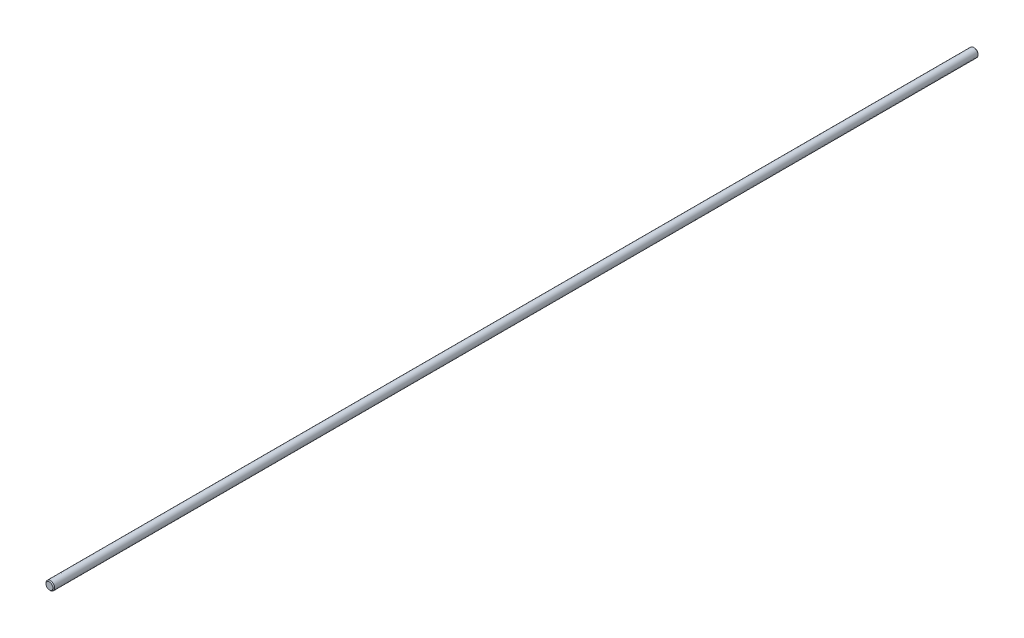
SolidWorks part; units mm, degrees
material "45#"
ref_plane "前基準面" through (0, 0, 0) normal (0, 0, 1) x (1, 0, 0)
ref_plane "上基準面" through (0, 0, 0) normal (0, 1, 0) x (1, 0, 0)
ref_plane "右基準面" through (0, 0, 0) normal (1, 0, 0) x (0, 0, -1)
sketch "草图1" plane through (0, 0, 0) normal (0, 0, 1) x (1, 0, 0)
  circle A0 centre (0, 0) radius 10
  dimension "D1" = 20
extrude "凸台-拉伸1" add sketch "草图1" along normal blind 2135
chamfer "倒角1" distance 2 angle 45 2 edges at (10, 0, 0) (10, 0, 2135)
